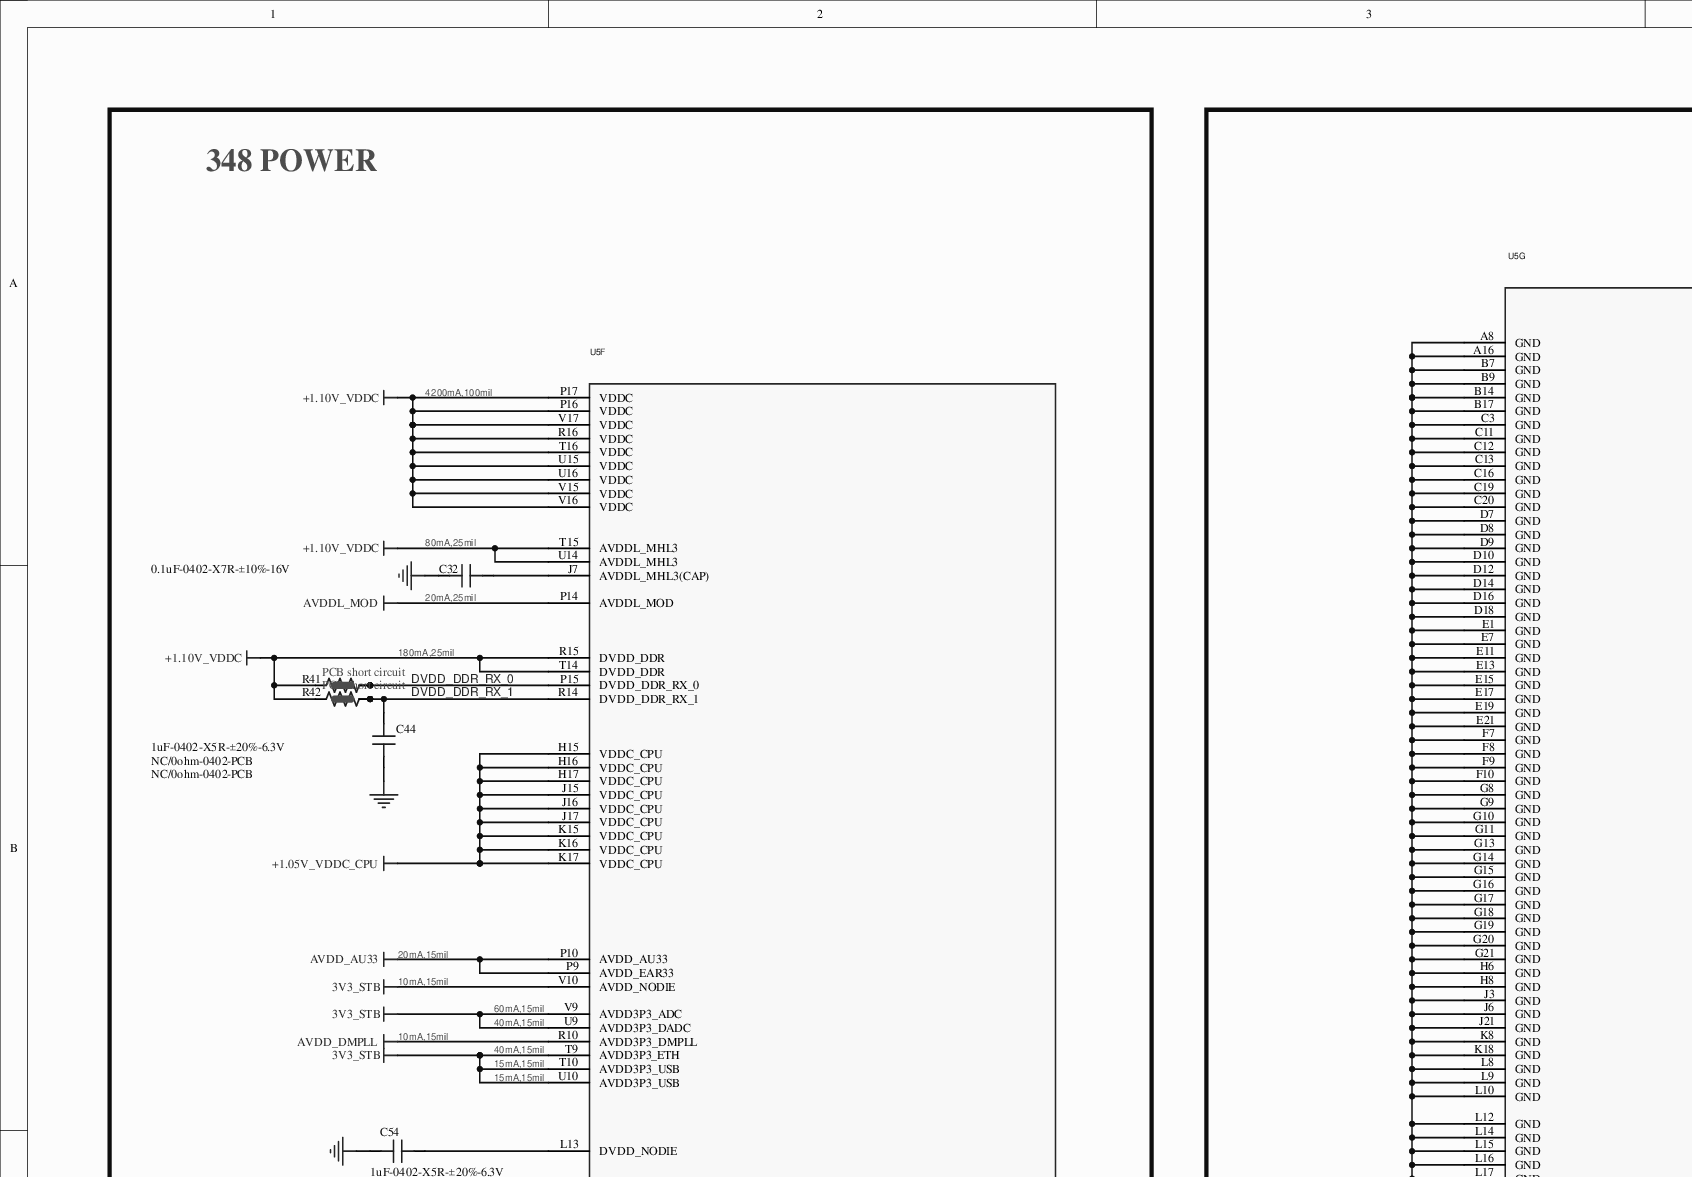
[diagram p0: MISC84395-9.SchDoc, top left]
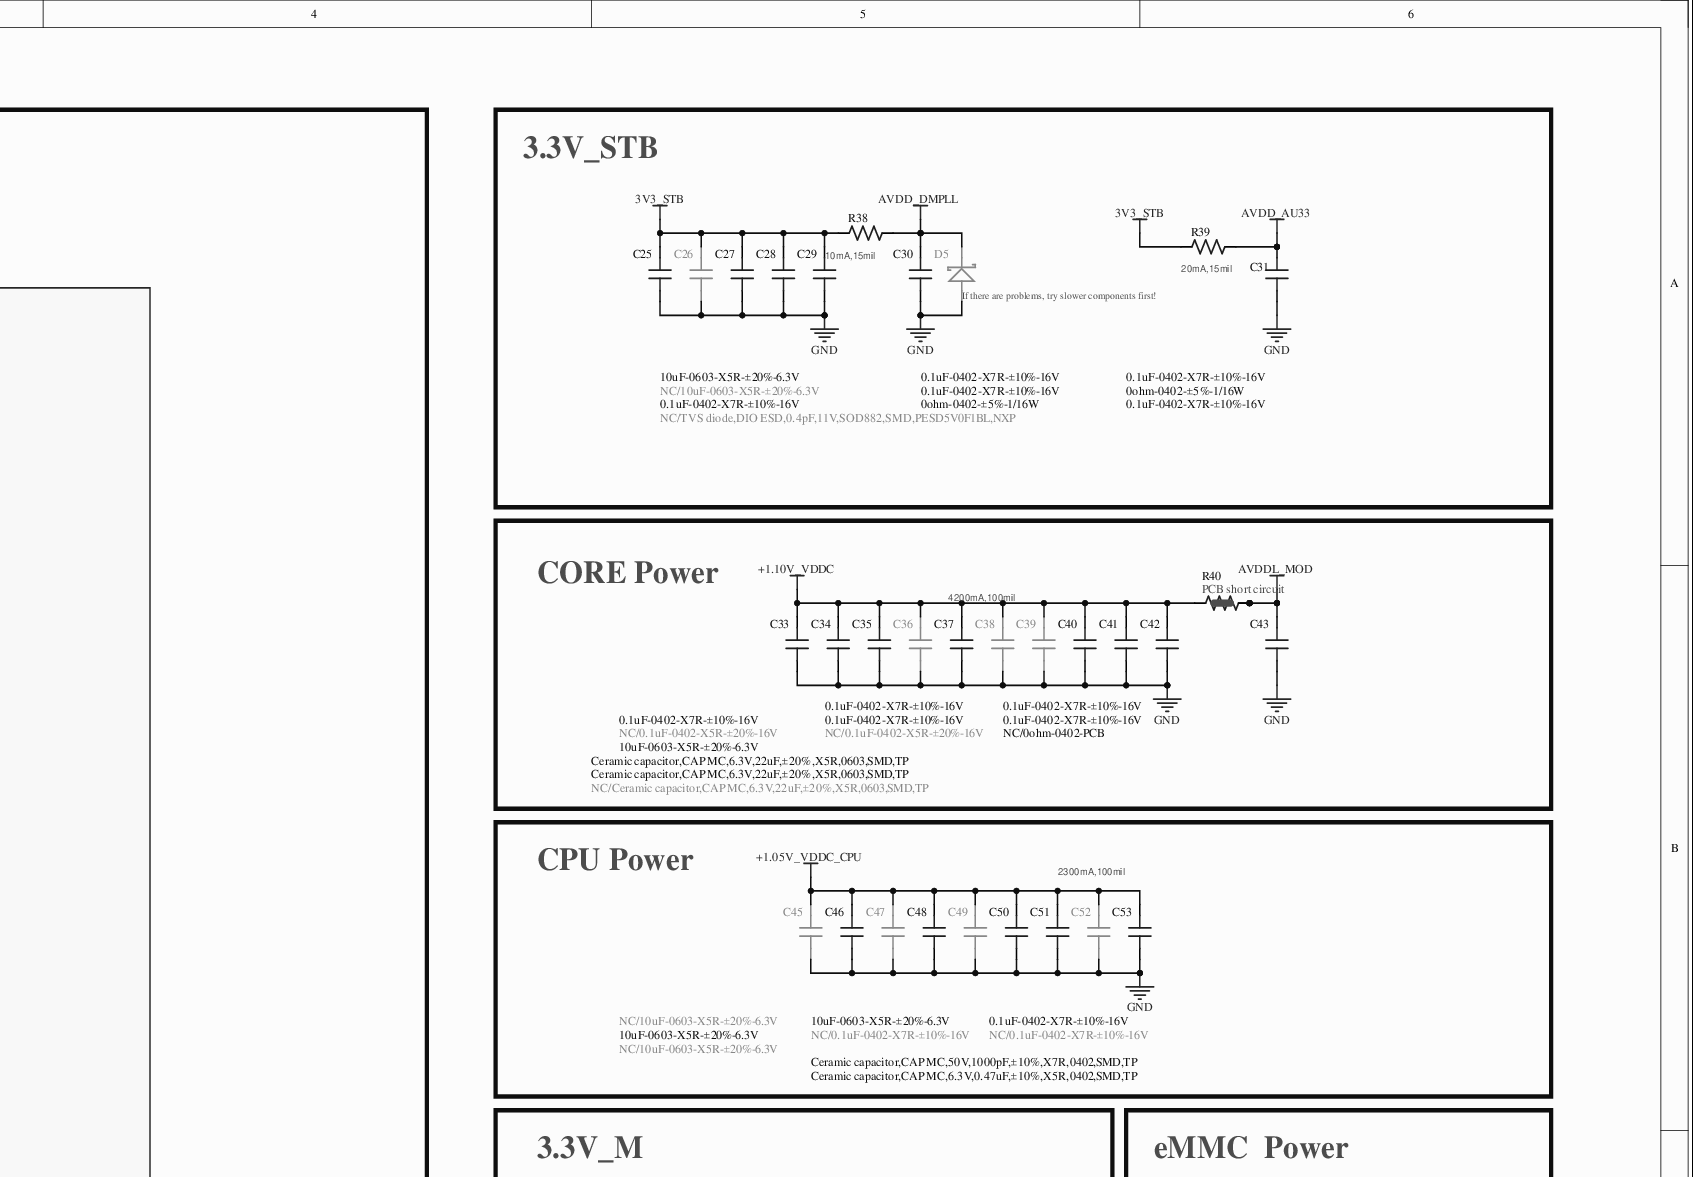
[diagram p1: MISC84395-9.SchDoc, top right]
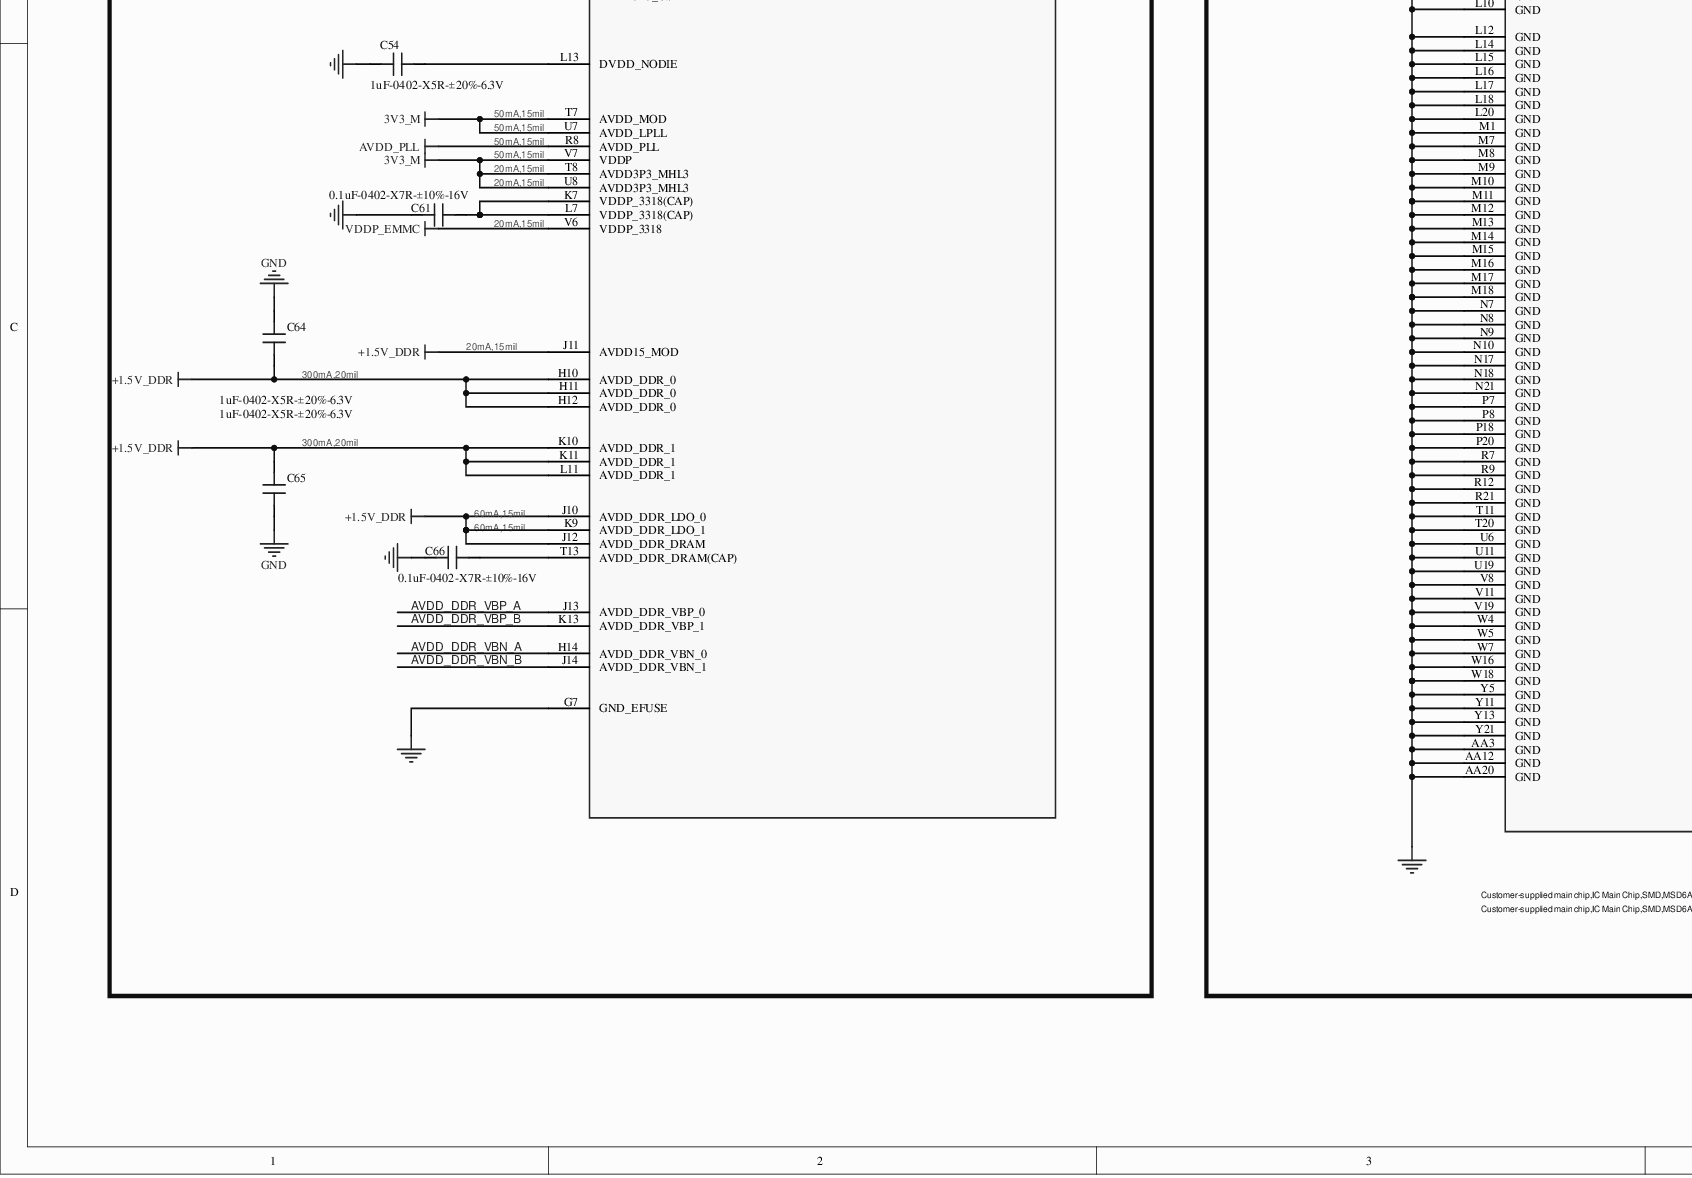
[diagram p2: MISC84395-9.SchDoc, bottom left]
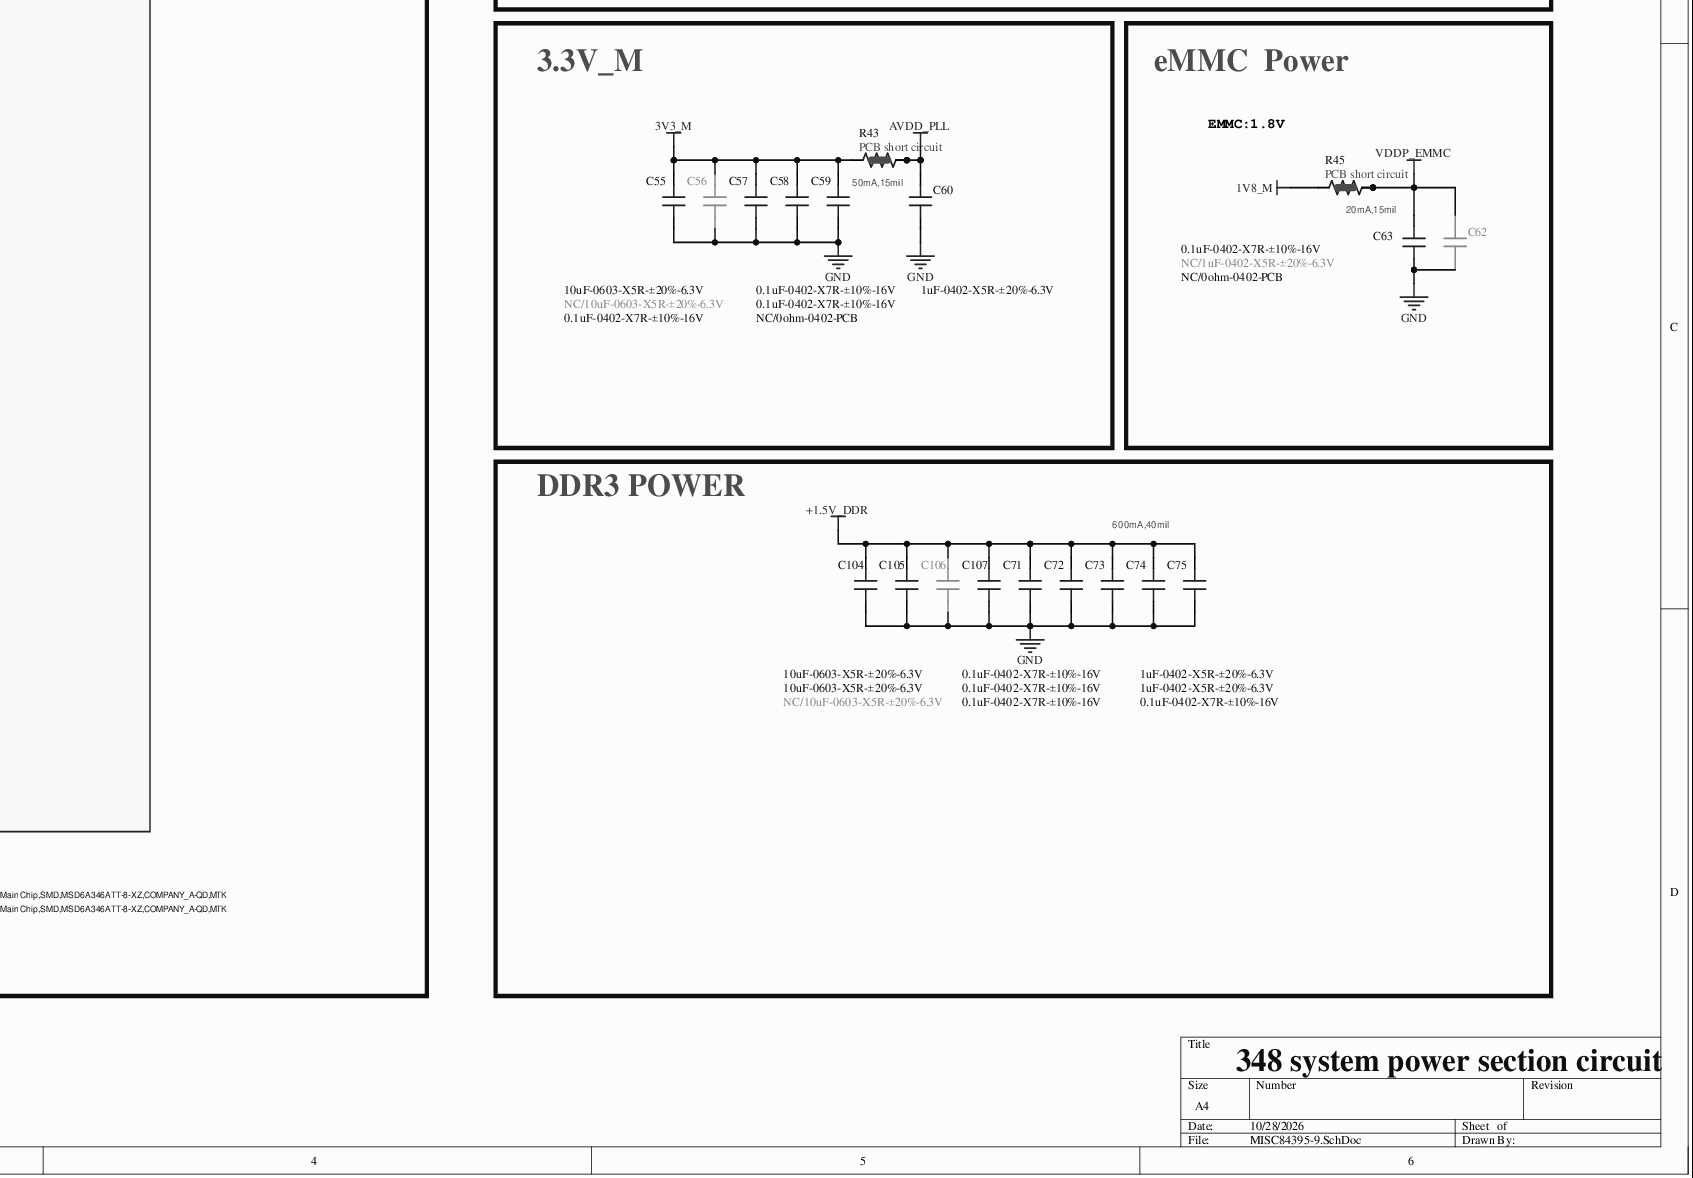
[diagram p3: MISC84395-9.SchDoc, bottom right]
# Altium project MISC84395-37.PrjPCB (part 6 of 13)

## Sheet MISC84395-9.SchDoc
size 609 x 419 mm

### Parts
C25  10uF-0603-X5R-±20%-6.3V  [C0603]
C26  NC/10uF-0603-X5R-±20%-6.3V  [C0603]
C27  0.1uF-0402-X7R-±10%-16V  [C0402]
C28  0.1uF-0402-X7R-±10%-16V  [C0402]
C29  0.1uF-0402-X7R-±10%-16V  [C0402]
C30  0.1uF-0402-X7R-±10%-16V  [C0402]
C31  0.1uF-0402-X7R-±10%-16V  [C0402]
C32  0.1uF-0402-X7R-±10%-16V  [C0402]
C33  10uF-0603-X5R-±20%-6.3V  [C0603]
C34  Ceramic capacitor,CAP MC,6.3V,22uF,±20%,X5R,0603,SMD,TP  [C0603]
C35  Ceramic capacitor,CAP MC,6.3V,22uF,±20%,X5R,0603,SMD,TP  [C0603]
C36  NC/Ceramic capacitor,CAP MC,6.3V,22uF,±20%,X5R,0603,SMD,TP  [C0603]
C37  0.1uF-0402-X7R-±10%-16V  [C0402]
C38  NC/0.1uF-0402-X5R-±20%-16V  [C0402]
C39  NC/0.1uF-0402-X5R-±20%-16V  [C0402]
C40  0.1uF-0402-X7R-±10%-16V  [C0402]
C41  0.1uF-0402-X7R-±10%-16V  [C0402]
C42  0.1uF-0402-X7R-±10%-16V  [C0402]
C43  0.1uF-0402-X7R-±10%-16V  [C0402]
C44  1uF-0402-X5R-±20%-6.3V  [C0402]
C45  NC/10uF-0603-X5R-±20%-6.3V  [C0603]
C46  10uF-0603-X5R-±20%-6.3V  [C0603]
C47  NC/10uF-0603-X5R-±20%-6.3V  [C0603]
C48  10uF-0603-X5R-±20%-6.3V  [C0603]
C49  NC/0.1uF-0402-X7R-±10%-16V  [C0402]
C50  Ceramic capacitor,CAP MC,50V,1000pF,±10%,X7R,0402,SMD,TP  [C0402]
C51  0.1uF-0402-X7R-±10%-16V  [C0402]
C52  NC/0.1uF-0402-X7R-±10%-16V  [C0402]
C53  Ceramic capacitor,CAP MC,6.3V,0.47uF,±10%,X5R,0402,SMD,TP  [C0402]
C54  1uF-0402-X5R-±20%-6.3V  [C0402]
C55  10uF-0603-X5R-±20%-6.3V  [C0603]
C56  NC/10uF-0603-X5R-±20%-6.3V  [C0603]
C57  0.1uF-0402-X7R-±10%-16V  [C0402]
C58  0.1uF-0402-X7R-±10%-16V  [C0402]
C59  0.1uF-0402-X7R-±10%-16V  [C0402]
C60  1uF-0402-X5R-±20%-6.3V  [C0402]
C61  0.1uF-0402-X7R-±10%-16V  [C0402]
C62  NC/1uF-0402-X5R-±20%-6.3V  [C0402]
C63  0.1uF-0402-X7R-±10%-16V  [C0402]
C64  1uF-0402-X5R-±20%-6.3V  [C0402]
C65  1uF-0402-X5R-±20%-6.3V  [C0402]
C66  0.1uF-0402-X7R-±10%-16V  [C0402]
C71  0.1uF-0402-X7R-±10%-16V  [C0402]
C72  0.1uF-0402-X7R-±10%-16V  [C0402]
C73  0.1uF-0402-X7R-±10%-16V  [C0402]
C74  1uF-0402-X5R-±20%-6.3V  [C0402]
C75  1uF-0402-X5R-±20%-6.3V  [C0402]
C104  10uF-0603-X5R-±20%-6.3V  [C0603]
C105  10uF-0603-X5R-±20%-6.3V  [C0603]
C106  NC/10uF-0603-X5R-±20%-6.3V  [C0603]
C107  0.1uF-0402-X7R-±10%-16V  [C0402]
D5  NC/TVS diode,DIO ESD,0.4pF,11V,SOD882,SMD,PESD5V0F1BL,NXP  [DIODE-S0402]
R38  0ohm-0402-±5%-1/16W  [R0402]
R39  0ohm-0402-±5%-1/16W  [R0402]
R40  NC/0ohm-0402-PCB  [R0402SC]
R41  NC/0ohm-0402-PCB  [R0402SC]
R42  NC/0ohm-0402-PCB  [R0402SC]
R43  NC/0ohm-0402-PCB  [R0402SC]
R45  NC/0ohm-0402-PCB  [R0402SC]
U5  Customer-supplied main chip,IC Main Chip,SMD,MSD6A346ATT-8-XZ,COMPANY_A-QD,MTK  [BGA406/0.8]  (parts F,G of 7)

### Blocks framed on the sheet
348 POWER: C32 C44 C54 C61 C64-C66 R41 R42 U5
3.3V_STB: C25-C31 D5 R38 R39
CORE Power: C33-C43 R40
CPU Power: C45-C53
3.3V_M: C55-C60 R43
eMMC  Power: C62 C63 R45
DDR3 POWER: C71-C75 C104-C107

### Nets
1V8_M: R45.1
3V3_M: C55.2 C56.2 C57.2 C58.2 C59.2 R43.1 U5.T7(AVDD_MOD) U5.T8(AVDD3P3_MHL3) U5.U7(AVDD_LPLL) U5.U8(AVDD3P3_MHL3) U5.V7(VDDP)
3V3_STB: C25.2 C26.2 C27.2 C28.2 C29.2 R38.1 R39.1 U5.T9(AVDD3P3_ETH) U5.T10(AVDD3P3_USB) U5.U9(AVDD3P3_DADC) U5.U10(AVDD3P3_USB) U5.V9(AVDD3P3_ADC) U5.V10(AVDD_NODIE)
+1.5V_DDR: C64.1 C65.2 C71.2 C72.2 C73.2 C74.2 C75.2 C104.2 C105.2 C106.2 C107.2 U5.H10(AVDD_DDR_0) U5.H11(AVDD_DDR_0) U5.H12(AVDD_DDR_0) U5.J10(AVDD_DDR_LDO_0) U5.J11(AVDD15_MOD) U5.J12(AVDD_DDR_DRAM) U5.K9(AVDD_DDR_LDO_1) U5.K10(AVDD_DDR_1) U5.K11(AVDD_DDR_1) U5.L11(AVDD_DDR_1)
+1.05V_VDDC_CPU: C45.2 C46.2 C47.2 C48.2 C49.2 C50.2 C51.2 C52.2 C53.2 U5.H15(VDDC_CPU) U5.H16(VDDC_CPU) U5.H17(VDDC_CPU) U5.J15(VDDC_CPU) U5.J16(VDDC_CPU) U5.J17(VDDC_CPU) U5.K15(VDDC_CPU) U5.K16(VDDC_CPU) U5.K17(VDDC_CPU)
+1.10V_VDDC: C33.2 C34.2 C35.2 C36.2 C37.2 C38.2 C39.2 C40.2 C41.2 C42.2 R40.1 R41.1 R42.1 U5.P16(VDDC) U5.P17(VDDC) U5.R15(DVDD_DDR) U5.R16(VDDC) U5.T14(DVDD_DDR) U5.T15(AVDDL_MHL3) U5.T16(VDDC) U5.U14(AVDDL_MHL3) U5.U15(VDDC) U5.U16(VDDC) U5.V15(VDDC) U5.V16(VDDC) U5.V17(VDDC)
AVDD_AU33: C31.2 R39.2 U5.P9(AVDD_EAR33) U5.P10(AVDD_AU33)
AVDD_DMPLL: C30.2 D5.K R38.2 U5.R10(AVDD3P3_DMPLL)
AVDD_PLL: C60.2 R43.2 R43.3 U5.R8(AVDD_PLL)
AVDDL_MOD: C43.2 R40.2 R40.3 U5.P14(AVDDL_MOD)
GND: C25.1 C26.1 C27.1 C28.1 C29.1 C30.1 C31.1 C32.1 C33.1 C34.1 C35.1 C36.1 C37.1 C38.1 C39.1 C40.1 C41.1 C42.1 C43.1 C44.1 C45.1 C46.1 C47.1 C48.1 C49.1 C50.1 C51.1 C52.1 C53.1 C54.2 C55.1 C56.1 C57.1 C58.1 C59.1 C60.1 C61.1 C62.1 C63.1 C64.2 C65.1 C66.2 C71.1 C72.1 C73.1 C74.1 C75.1 C104.1 C105.1 C106.1 C107.1 D5.A U5.A8(GND) U5.A16(GND) U5.AA3(GND) U5.AA12(GND) U5.AA20(GND) U5.B7(GND) U5.B9(GND) U5.B14(GND) U5.B17(GND) U5.C3(GND) U5.C11(GND) U5.C12(GND) U5.C13(GND) U5.C16(GND) U5.C19(GND) U5.C20(GND) U5.D7(GND) U5.D8(GND) U5.D9(GND) U5.D10(GND) U5.D12(GND) U5.D14(GND) U5.D16(GND) U5.D18(GND) U5.E1(GND) U5.E7(GND) U5.E11(GND) U5.E13(GND) U5.E15(GND) U5.E17(GND) U5.E19(GND) U5.E21(GND) U5.F7(GND) U5.F8(GND) U5.F9(GND) U5.F10(GND) U5.G7(GND_EFUSE) U5.G8(GND) U5.G9(GND) U5.G10(GND) U5.G11(GND) U5.G13(GND) U5.G14(GND) U5.G15(GND) U5.G16(GND) U5.G17(GND) U5.G18(GND) U5.G19(GND) U5.G20(GND) U5.G21(GND) U5.H6(GND) U5.H8(GND) U5.J3(GND) U5.J6(GND) U5.J21(GND) U5.K8(GND) U5.K18(GND) U5.L8(GND) U5.L9(GND) U5.L10(GND) U5.L12(GND) U5.L14(GND) U5.L15(GND) U5.L16(GND) U5.L17(GND) U5.L18(GND) U5.L20(GND) U5.M1(GND) U5.M7(GND) U5.M8(GND) U5.M9(GND) U5.M10(GND) U5.M11(GND) U5.M12(GND) U5.M13(GND) U5.M14(GND) U5.M15(GND) U5.M16(GND) U5.M17(GND) U5.M18(GND) U5.N7(GND) U5.N8(GND) U5.N9(GND) U5.N10(GND) U5.N17(GND) U5.N18(GND) U5.N21(GND) U5.P7(GND) U5.P8(GND) U5.P18(GND) U5.P20(GND) U5.R7(GND) U5.R9(GND) U5.R12(GND) U5.R21(GND) U5.T11(GND) U5.T20(GND) U5.U6(GND) U5.U11(GND) U5.U19(GND) U5.V8(GND) U5.V11(GND) U5.V19(GND) U5.W4(GND) U5.W5(GND) U5.W7(GND) U5.W16(GND) U5.W18(GND) U5.Y5(GND) U5.Y11(GND) U5.Y13(GND) U5.Y21(GND)
VDDP_EMMC: C62.2 C63.2 R45.2 R45.3 U5.V6(VDDP_3318)
AVDD_DDR_VBN_A: U5.H14(AVDD_DDR_VBN_0)
AVDD_DDR_VBN_B: U5.J14(AVDD_DDR_VBN_1)
AVDD_DDR_VBP_A: U5.J13(AVDD_DDR_VBP_0)
AVDD_DDR_VBP_B: U5.K13(AVDD_DDR_VBP_1)
DVDD_DDR_RX_0: R41.2 R41.3 U5.P15(DVDD_DDR_RX_0)
DVDD_DDR_RX_1: C44.2 R42.2 R42.3 U5.R14(DVDD_DDR_RX_1)
NetC32_2: C32.2 U5.J7(AVDDL_MHL3(CAP))
NetC54_1: C54.1 U5.L13(DVDD_NODIE)
NetC61_2: C61.2 U5.K7(VDDP_3318(CAP)) U5.L7(VDDP_3318(CAP))
NetC66_1: C66.1 U5.T13(AVDD_DDR_DRAM(CAP))

### Notes on the sheet
- (near C29) 10mA,15mil
- (near D5) If there are problems, try slower components first!
- (near R39) 20mA,15mil
- 4200mA,100mil
- (near C32) 80mA,25mil
- (near C32) 20mA,25mil
- 180mA,25mil
- 2300mA,100mil
- 20mA,15mil
- 10mA,15mil
- (near U5) 60mA,15mil
- (near U5) 40mA,15mil
- (near U5) 15mA,15mil
- (near U5) 50mA,15mil
- 50mA,15mil
- (near R45) EMMC:1.8V
- (near C64) 300mA,20mil
- (near C65) 300mA,20mil
- (near C66) 60mA,15mil
- 600mA,40mil
- 348 system power section circuit

### Library data of the parts
C25 C26 C33-C36 C45-C48 C55 C56 C104-C106 = 10uF-0603-X5R-±20%-6.3V-D
C27-C31 C37-C43 C49-C53 C57-C59 C63 C71-C73 C107 = 0.1uF-0402-X7R-±10%-16V-D
C32 C61 C66 = 0.1uF-0402-X5R-±20%-16V-D
C44 C54 C60 C62 C74 C75 = 1uF-0402-X5R-±20%-6.3V-D
C64 C65 = 2.2uF-0402-X5R-±20%-6.3V-D
D5 = SFI0402-240E-2R5PP-LF-D
R38 R39 = 0ohm-0402-±5%-1/16W-D
R40-R43 R45 = 0ohm-0402-PCB-D
U5 = 004.016.0000830: TV main chip,IC Main Chip,MSD6A348AT-X1,CAN TV,32bit,Multi-Core,BGA406,SMD,Mstar-D